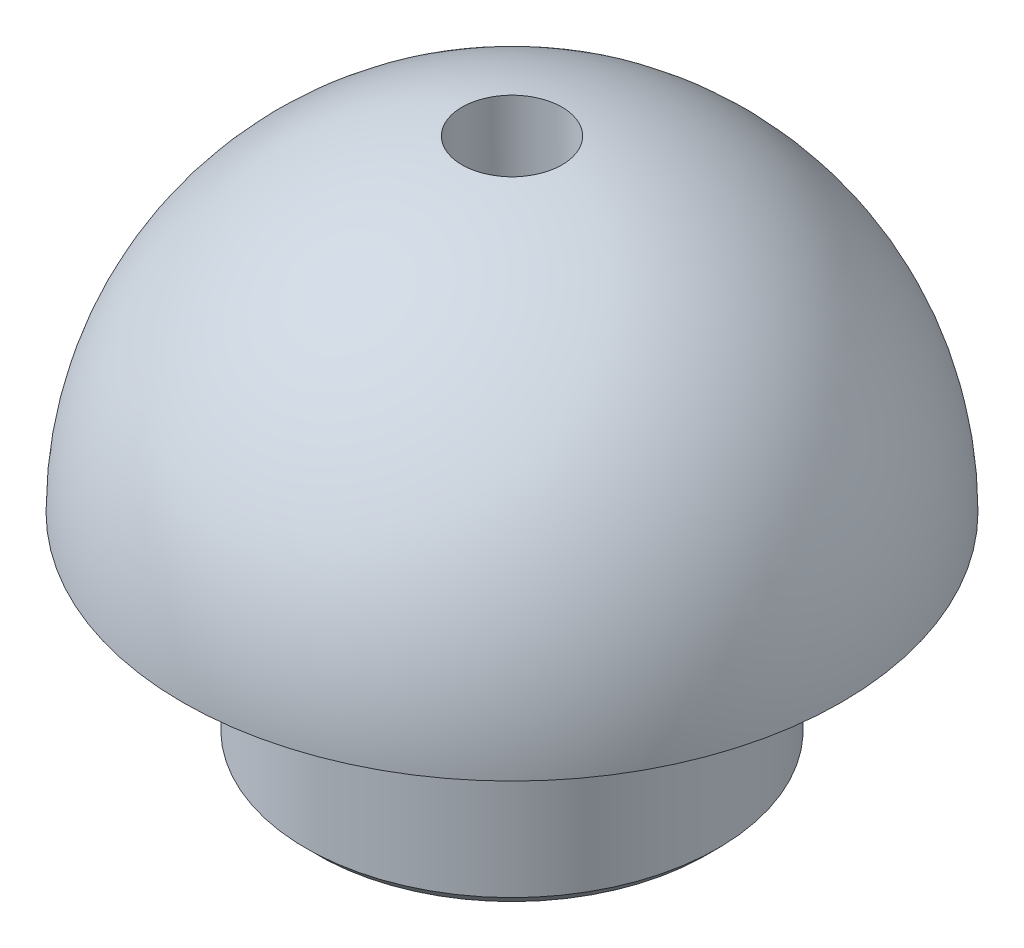
from build123d import *

# Parameters (mm, degrees)
HOLE_WIZARD_M10_1_D     = 8.5
HOLE_WIZARD_M10_1_DEPTH = 12
HOLE_WIZARD_M10_1_TIP   = 2.553657631
CHAMFER_1_SIZE          = 1


with BuildPart() as part:
    # 草图1 → 旋转1 (revolve)
    with BuildSketch(Plane.XY, mode=Mode.PRIVATE) as revolve_1_sk:
        with BuildLine():
            Line((17.5, 0), (28, 0))
            ThreePointArc((28, 0), (19.798989873, 19.798989873), (0, 28))
            Line((0, 28), (0, 0))
            Line((0, 0), (0, -17))
            Line((0, -17), (17.5, -17))
            Line((17.5, -17), (17.5, 0))
        make_face()
    revolve(revolve_1_sk.sketch.rotate(Axis((0, 0, 0), (0, 1, 0)), 90), axis=Axis((0, 0, 0), (0, 1, 0)))

    # M10 螺纹孔1
    with Locations(Plane(origin=(0, 28, 0), x_dir=(1, 0, 0), z_dir=(0, 1, 0))):
        with Locations((0, 0)):
            Hole(HOLE_WIZARD_M10_1_D / 2, depth=HOLE_WIZARD_M10_1_DEPTH)
            with Locations((0, 0, -(HOLE_WIZARD_M10_1_DEPTH + HOLE_WIZARD_M10_1_TIP / 2))):  # 118° drill point
                Cone(0, HOLE_WIZARD_M10_1_D / 2, HOLE_WIZARD_M10_1_TIP, mode=Mode.SUBTRACT)

    # 倒角1
    chamfer_1_edges = [part.edges().sort_by_distance(p)[0] for p in [
        (0, -17, 17.5),
    ]]
    chamfer(chamfer_1_edges, length=CHAMFER_1_SIZE)


solid = part.part
